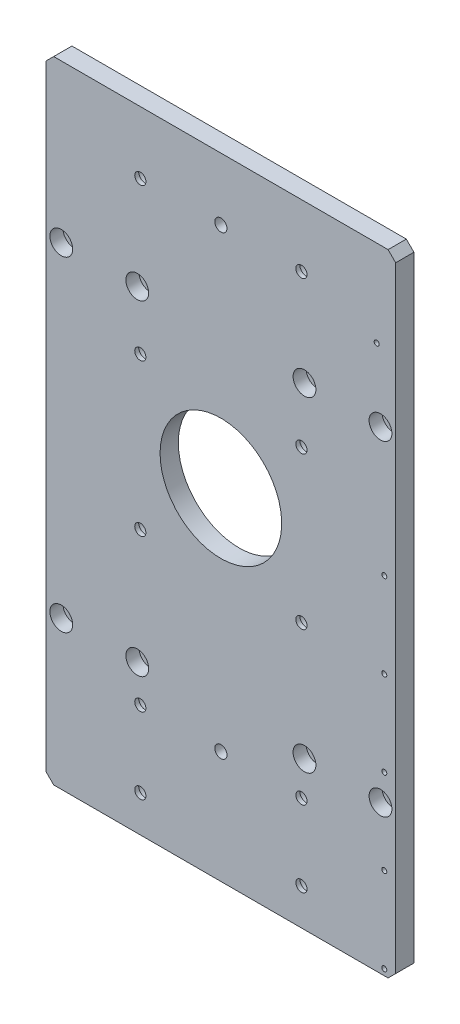
SolidWorks part; units mm, degrees
material "6061-T6"
ref_plane "前视基准面" through (0, 0, 0) normal (0, 0, 1) x (1, 0, 0)
ref_plane "上视基准面" through (0, 0, 0) normal (0, 1, 0) x (1, 0, 0)
ref_plane "右视基准面" through (0, 0, 0) normal (1, 0, 0) x (0, 0, -1)
sketch "草图1" plane through (0, 0, 0) normal (0, 0, 1) x (1, 0, 0)
  line L1 (210.0261, 629.8574) -> (-19.9739, 629.8574)
  line L2 (210.0261, 629.8574) -> (210.0261, 214.8574)
  line L3 (210.0261, 214.8574) -> (-19.9739, 214.8574)
  line L4 (-19.9739, 629.8574) -> (-19.9739, 214.8574)
  dimension "D1" = 230
  dimension "D2" = 415
extrude "凸台-拉伸1" add sketch "草图1" along normal blind 12
chamfer "倒角1" distance 5 angle 45 4 edges at (-19.9739, 214.8574, 6) (210.0261, 214.8574, 6) (210.0261, 629.8574, 6) (-19.9739, 629.8574, 6)
hole_wizard "M8 六角凹头螺钉的柱形沉头孔1" positions "草图2" profile "草图3" counterbore size "M8" standard "ISO"
sketch "草图2" plane through (0, 0, 0) normal (0, 0, -1) x (-1, 0, 0)
  point P0 (-148.0261, 588.8574)
  point P2 (-42.0261, 588.8574)
  point P4 (-148.0261, 488.8574)
  point P6 (-42.0261, 488.8574)
  point P8 (-148.0261, 388.8574)
  point P10 (-42.0261, 388.8574)
  point P12 (-148.0261, 288.8574)
  point P14 (-42.0261, 288.8574)
  point P16 (-148.0261, 238.8574)
  point P18 (-42.0261, 238.8574)
sketch "草图3" plane through (148.0261, 588.8574, 0) normal (1, 0, 0) x (0, 1, 0)
  line L0 (0, 0) -> (0, 14.2039)
  line L1 (0, 14.2039) -> (4.5, 11.5)
  line L2 (4.5, 11.5) -> (4.5, 8.6)
  line L3 (4.5, 8.6) -> (7.5, 8.6)
  line L4 (7.5, 8.6) -> (7.5, 0)
  line L5 (7.5, 0) -> (0, 0)
  line L10 (0, 14.2039) -> (-4.5, 11.5) construction
  line L11 (0, -6.35) -> (0, 107.95) construction
  dimension "孔直径" = 9
  dimension "孔深度" = 11.5
  dimension "柱形沉头孔直径" = 15
  dimension "柱形沉头孔深度" = 8.6
  dimension "导头角度" = 118
hole_wizard "M8 六角凹头螺钉的柱形沉头孔2" positions "草图4" profile "草图5" counterbore size "M8" standard "ISO"
sketch "草图4" plane through (0, 0, 12) normal (0, 0, 1) x (1, 0, 0)
  line L0 (210.0261, 419.3574) -> (254.3522, 419.3574) construction
  point P0 (-9.9739, 526.3574)
  point P2 (40.0261, 526.3574)
  point P6 (150.0261, 526.3574)
  point P8 (200.0261, 526.3574)
  point P16 (200.0261, 312.3574)
  point P17 (150.0261, 312.3574)
  point P19 (40.0261, 312.3574)
  point P20 (-9.9739, 312.3574)
sketch "草图5" plane through (-9.9739, 526.3574, 12) normal (1, 0, 0) x (0, -1, 0)
  line L0 (0, 0) -> (0, 24.9539)
  line L1 (0, 24.9539) -> (4.5, 22.25)
  line L2 (4.5, 22.25) -> (4.5, 8.6)
  line L3 (4.5, 8.6) -> (7.5, 8.6)
  line L4 (7.5, 8.6) -> (7.5, 0)
  line L5 (7.5, 0) -> (0, 0)
  line L10 (0, 24.9539) -> (-4.5, 22.25) construction
  line L11 (0, -6.35) -> (0, 107.95) construction
  dimension "孔直径" = 9
  dimension "孔深度" = 22.25
  dimension "柱形沉头孔直径" = 15
  dimension "柱形沉头孔深度" = 8.6
  dimension "导头角度" = 118
hole_wizard "大小mm 暗销孔1" positions "草图6" profile "草图7" hole size "Ø8.0" standard "ISO"
sketch "草图6" plane through (0, 0, 12) normal (0, 0, 1) x (1, 0, 0)
  point P0 (95.0261, 588.8574)
  point P2 (95.0261, 288.8574)
sketch "草图7" plane through (95.0261, 588.8574, 12) normal (1, 0, 0) x (0, -1, 0)
  line L0 (0, 0) -> (0, 24.6534)
  line L1 (0, 24.6534) -> (4, 22.25)
  line L2 (4, 22.25) -> (4, 0)
  line L5 (4, 0) -> (0, 0)
  line L10 (0, 24.6534) -> (-4, 22.25) construction
  line L11 (0, -6.35) -> (0, 107.95) construction
  dimension "孔直径" = 8
  dimension "孔深度" = 22.25
  dimension "导头角度" = 118
hole_wizard "M4 螺纹孔1" positions "草图8" profile "草图9" tap size "M4" standard "ISO" end condition through all
sketch "草图8" plane through (0, 0, 12) normal (0, 0, 1) x (1, 0, 0)
  point P0 (202.5261, 218.8574)
  point P2 (202.5261, 274.8574)
  point P4 (202.5261, 330.8574)
  point P6 (202.5261, 386.8574)
  point P8 (202.5261, 442.8574)
cosmetic thread "孔螺蚊线1" parameters "D2"=4
cosmetic thread "孔螺蚊线2" parameters "D2"=4
cosmetic thread "孔螺蚊线3" parameters "D2"=4
cosmetic thread "孔螺蚊线4" parameters "D2"=4
cosmetic thread "孔螺蚊线5" parameters "D2"=4
sketch "草图9" plane through (202.5261, 218.8574, 12) normal (1, 0, 0) x (0, -1, 0)
  line L0 (0, 0) -> (0, 12)
  line L1 (0, 12) -> (1.65, 12)
  line L2 (1.65, 12) -> (1.65, 0)
  line L5 (1.65, 0) -> (0, 0)
  line L11 (0, -6.35) -> (0, 107.95) construction
  dimension "通孔螺纹孔钻头直径" = 3.3
  dimension "通孔螺纹孔钻头深度" = 12
hole_wizard "M4 螺纹孔2" positions "草图10" profile "草图11" tap size "M4" standard "ISO" end condition through all
sketch "草图10" plane through (0, 0, 12) normal (0, 0, 1) x (1, 0, 0)
  point P0 (197.5261, 572.8574)
sketch "草图11" plane through (197.5261, 572.8574, 12) normal (1, 0, 0) x (0, -1, 0)
  line L0 (0, 0) -> (0, 12)
  line L1 (0, 12) -> (1.65, 12)
  line L2 (1.65, 12) -> (1.65, 0)
  line L5 (1.65, 0) -> (0, 0)
  line L11 (0, -6.35) -> (0, 107.95) construction
  dimension "通孔螺纹孔钻头直径" = 3.3
  dimension "通孔螺纹孔钻头深度" = 12
cosmetic thread "孔螺蚊线6" parameters "D2"=4
sketch "草图12" plane through (0, 0, 0) normal (0, 0, -1) x (-1, 0, 0)
  line L0 (-148.0261, 488.8574) -> (-42.0261, 388.8574) construction
  circle A0 centre (-95.0261, 438.8574) radius 40
  dimension "D1" = 80
extrude "切除-拉伸1" cut sketch "草图12" against normal through all
